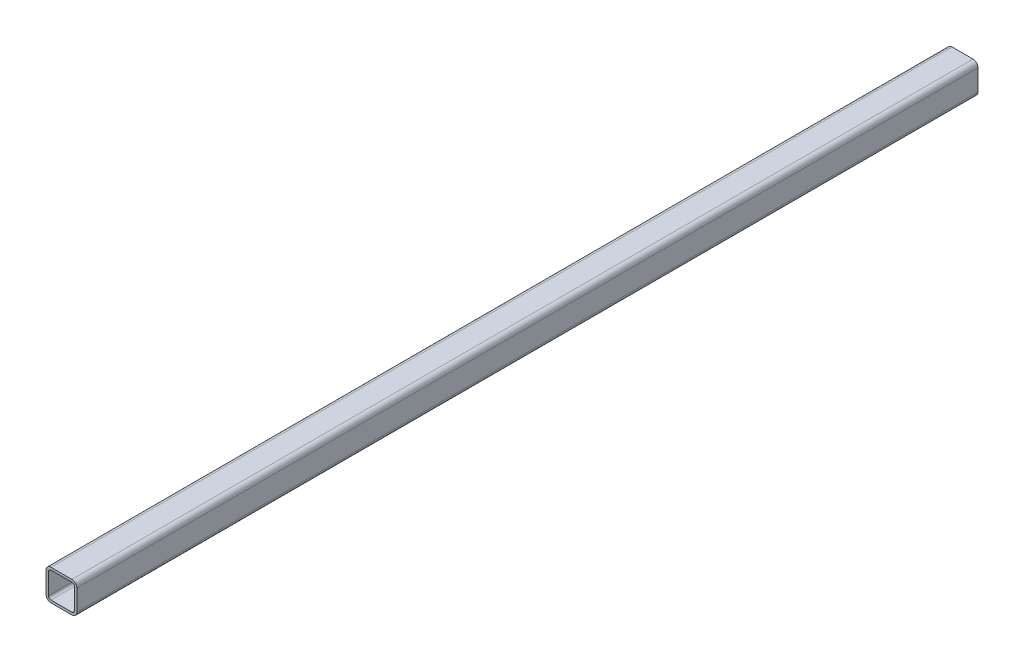
from build123d import *

# Parameters (mm, degrees)
BOSS_EXTRUDE1_DEPTH = 730


with BuildPart() as part:
    # Sketch1 → Boss-Extrude1 (new body)
    with BuildSketch(Plane.XY):
        with BuildLine():
            Line((-8.5, -12.5), (8.5, -12.5))
            ThreePointArc((8.5, -12.5), (11.328427125, -11.328427125), (12.5, -8.5))
            Line((12.5, -8.5), (12.5, 8.5))
            ThreePointArc((12.5, 8.5), (11.328427125, 11.328427125), (8.5, 12.5))
            Line((8.5, 12.5), (-8.5, 12.5))
            ThreePointArc((-8.5, 12.5), (-11.328427125, 11.328427125), (-12.5, 8.5))
            Line((-12.5, 8.5), (-12.5, -8.5))
            ThreePointArc((-12.5, -8.5), (-11.328427125, -11.328427125), (-8.5, -12.5))
        make_face()
        with BuildLine():
            Line((-8.5, -10.5), (8.5, -10.5))
            ThreePointArc((8.5, -10.5), (9.914213562, -9.914213562), (10.5, -8.5))
            Line((10.5, -8.5), (10.5, 8.5))
            ThreePointArc((10.5, 8.5), (9.914213562, 9.914213562), (8.5, 10.5))
            Line((8.5, 10.5), (-8.5, 10.5))
            ThreePointArc((-8.5, 10.5), (-9.914213562, 9.914213562), (-10.5, 8.5))
            Line((-10.5, 8.5), (-10.5, -8.5))
            ThreePointArc((-10.5, -8.5), (-9.914213562, -9.914213562), (-8.5, -10.5))
        make_face(mode=Mode.SUBTRACT)
    extrude(amount=BOSS_EXTRUDE1_DEPTH)


solid = part.part
